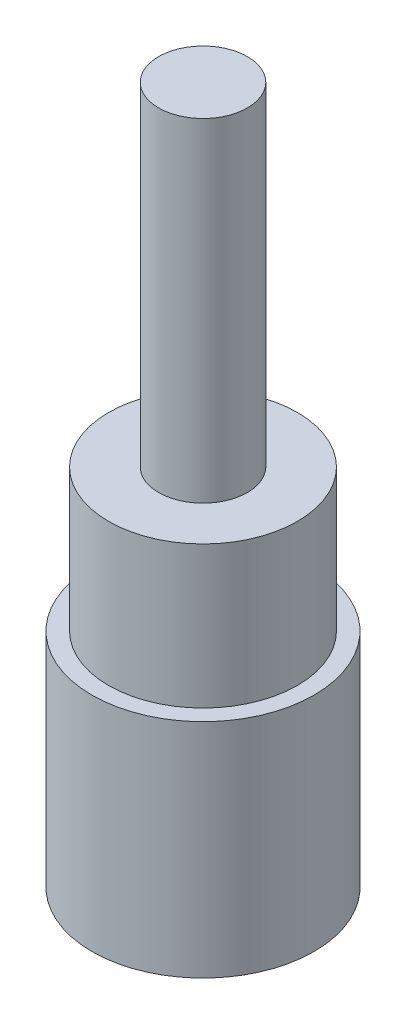
SolidWorks part; units mm, degrees
material "6061-T6 (SS)"
ref_plane "Front Plane" through (0, 0, 0) normal (0, 0, 1) x (1, 0, 0)
ref_plane "Top Plane" through (0, 0, 0) normal (0, 1, 0) x (1, 0, 0)
ref_plane "Right Plane" through (0, 0, 0) normal (1, 0, 0) x (0, 0, -1)
sketch "Sketch1" plane through (0, 0, 0) normal (0, 1, 0) x (1, 0, 0)
  circle A0 centre (0, 0) radius 10
  dimension "D1" = 20
extrude "Boss-Extrude1" add sketch "Sketch1" along normal blind 20
sketch "Sketch2" plane through (0, 20, 0) normal (0, 1, 0) x (1, 0, 0)
  circle A0 centre (0, 0) radius 8.5
  dimension "D1" = 17
extrude "Boss-Extrude2" add sketch "Sketch2" along normal blind 12.8
sketch "Sketch3" plane through (0, 32.8, 0) normal (0, 1, 0) x (1, 0, 0)
  circle A0 centre (0, 0) radius 4
  dimension "D1" = 8
extrude "Boss-Extrude3" add sketch "Sketch3" along normal blind 30
cosmetic thread "Cosmetic Thread1" parameters "D1"=10, "D2"=6.647
ref_plane "Plane1" through (0, 0, -4) normal (0, 0, -1) x (-1, 0, 0)
sketch "Sketch4" plane through (0, 0, -4) normal (0, 0, -1) x (-1, 0, 0)
  line L0 (0, 49.8) -> (0, 35.8) construction
  line L1 (1, 49.8) -> (1, 35.8)
  line L2 (-1, 49.8) -> (-1, 35.8)
  line L3 (8.5, 32.8) -> (-8.5, 32.8) construction
  arc A0 (1, 49.8) -> (-1, 49.8) centre (0, 49.8) ccw
  arc A1 (-1, 35.8) -> (1, 35.8) centre (0, 35.8) ccw
  point P3 (0, 42.8)
  dimension "D2" = 14
  dimension "D3" = 3
  dimension "D1" = 2
extrude "Cut-Extrude1" cut sketch "Sketch4" against normal blind 1.2
